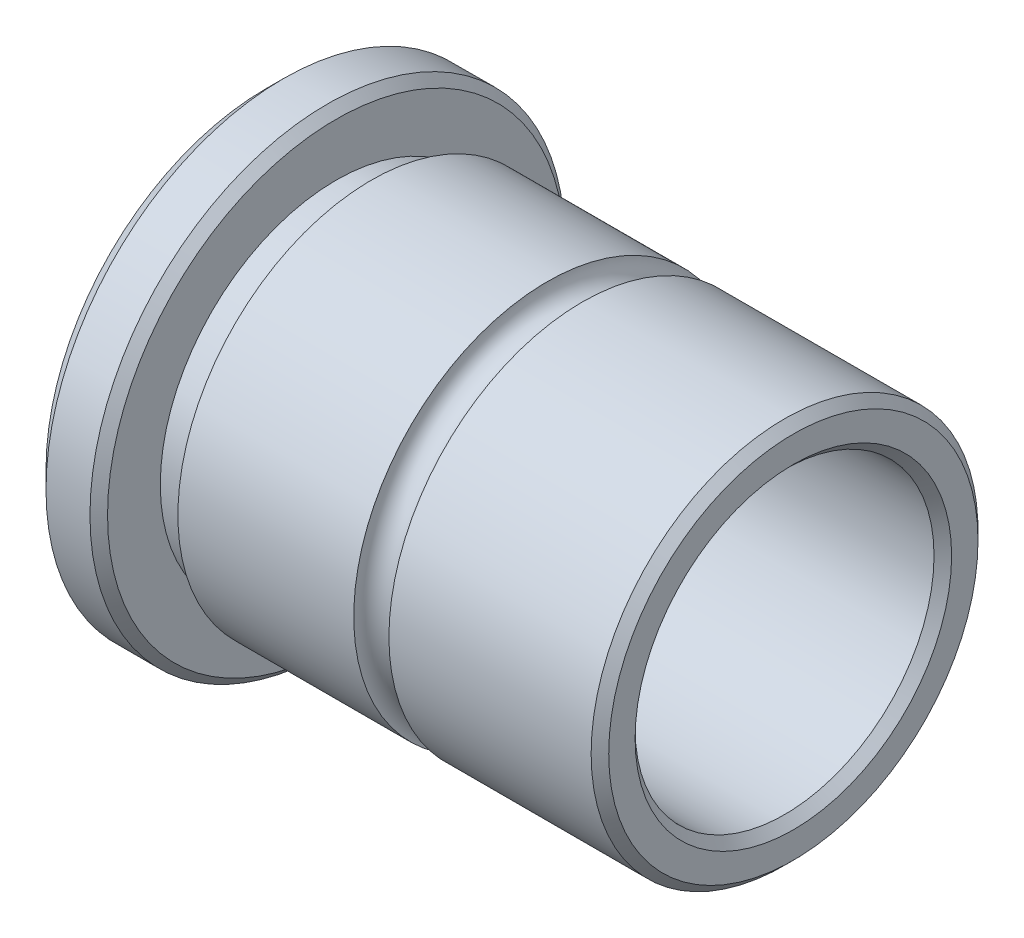
SolidWorks part; units mm, degrees
ref_plane "Front Plane" through (0, 0, 0) normal (0, 0, 1) x (1, 0, 0)
ref_plane "Top Plane" through (0, 0, 0) normal (0, 1, 0) x (1, 0, 0)
ref_plane "Right Plane" through (0, 0, 0) normal (1, 0, 0) x (0, 0, -1)
sketch "Sketch1" plane through (0, 0, 0) normal (0, 0, 1) x (1, 0, 0)
  line L0 (0, 0) -> (111.0846, 0) construction
  line L1 (30, 8.5) -> (0, 8.5)
  line L2 (0, 8.5) -> (0, 13.5)
  line L3 (0, 13.5) -> (4, 13.5)
  line L4 (4, 13.5) -> (4, 11)
  line L5 (4, 11) -> (30, 11)
  line L6 (30, 11) -> (30, 8.5)
  dimension "D1" = 22
  dimension "D2" = 27
  dimension "D3" = 17
  dimension "D4" = 4
  dimension "D5" = 30
revolve "Revolve1" add sketch "Sketch1" angle 360 about L0
chamfer "Chamfer1" distance 1 angle 45 1 edges at (0, 0, 13.5)
chamfer "Chamfer2" distance 0.5 angle 45 4 edges at (4, 0, 13.5) (0, 0, 8.5) (30, 0, 8.5) (30, 0, 11)
ref_axis "Axis1" through (29.5, 0, 0) along (-1, 0, 0)
sketch "Sketch2" plane through (0, 0, 0) normal (0, 1, 0) x (1, 0, 0)
  line L0 (29.5, 11) -> (4, 11) construction
  line L1 (29.5, 11) -> (4, 11) construction
  line L2 (4, 11) -> (4, 10)
  line L3 (4, -13) -> (4, 13) construction
  line L4 (4, 10) -> (5.8, 10)
  line L5 (5.8, 10) -> (6, 11)
  line L6 (29.5, 11) -> (4, 11) construction
  line L7 (6, 11) -> (4, 11)
  line L8 (29.5, 11) -> (4, 11) construction
  line L9 (0, 12.5) -> (0, -12.5) construction
  circle A0 centre (32, 11) radius 1
  circle A1 centre (17, 11) radius 1
  dimension "D1" = 2
  dimension "D2" = 2
  dimension "D3" = 1.8
  dimension "D4" = 17
revolve "Cut-Revolve1" cut sketch "Sketch2" angle 360 about axis through (29.5, 0, 0) along (-1, 0, 0)
